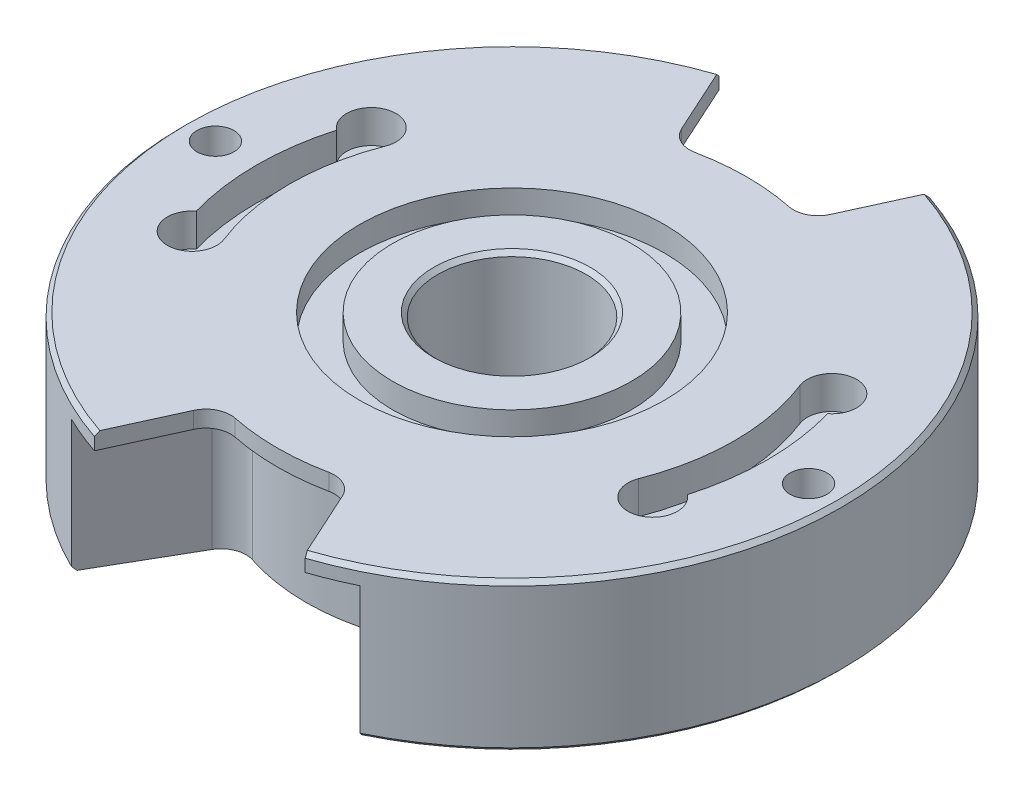
SolidWorks part; units mm, degrees
ref_plane "Front Plane" through (0, 0, 0) normal (0, 0, 1) x (1, 0, 0)
ref_plane "Top Plane" through (0, 0, 0) normal (0, 1, 0) x (1, 0, 0)
ref_plane "Right Plane" through (0, 0, 0) normal (1, 0, 0) x (0, 0, -1)
other "Configuration Table"
sketch "Sketch1" plane through (0, 0, 0) normal (0, 1, 0) x (1, 0, 0)
  circle A0 centre (0, 0) radius 40
  dimension "D1" = 80
extrude "Boss-Extrude1" add sketch "Sketch1" along normal blind 18
chamfer "Chamfer2" distance 0.5 angle 45 2 edges at (0, 0, 40) (0, 18, 40)
sketch "Sketch2" plane through (0, 18, 0) normal (0, 1, 0) x (1, 0, 0)
  line L0 (-36, 0) -> (36, 0) construction
  line L1 (0, 0) -> (0, -31.9265) construction
  circle A0 centre (36, 0) radius 2.25
  circle A1 centre (-36, 0) radius 2.25
  dimension "D1" = 4.5
  dimension "D2" = 36
extrude "Cut-Extrude1" cut sketch "Sketch2" against normal through all and the other way through all
sketch "Sketch3" plane through (0, 18, 0) normal (0, 1, 0) x (1, 0, 0)
  line L0 (-54.6069, 0) -> (54.6069, 0) construction
  line L1 (0, 0) -> (-45.6722, 23.2711) construction
  line L2 (0, 0) -> (-45.6722, -23.2711) construction
  line L3 (0, 0) -> (0, 53.5192) construction
  line L4 (0, 0) -> (45.6722, -23.2711) construction
  line L5 (0, 0) -> (45.6722, 23.2711) construction
  arc A0 (-25.1624, 9.7906) -> (-25.1624, -9.7906) centre (0, 0) ccw
  arc A2 (-25.1624, 9.7906) -> (-29.8073, 8.5161) centre (-27.9582, 10.8784) ccw
  arc A3 (-29.8073, 8.5161) -> (-29.8073, -8.5161) centre (0, 0) ccw
  arc A4 (-25.1624, -9.7906) -> (-29.8073, -8.5161) centre (-27.9582, -10.8784) cw
  arc A5 (25.1624, -9.7906) -> (29.8073, -8.5161) centre (27.9582, -10.8784) ccw
  arc A6 (29.8073, 8.5161) -> (29.8073, -8.5161) centre (0, 0) cw
  arc A7 (25.1624, 9.7906) -> (29.8073, 8.5161) centre (27.9582, 10.8784) cw
  arc A8 (25.1624, 9.7906) -> (25.1624, -9.7906) centre (0, 0) cw
  dimension "D1" = 54
  dimension "D2" = 31
  dimension "D4" = 6
  dimension "D3" = 27
extrude "Cut-Extrude2" cut sketch "Sketch3" against normal blind 4
sketch "Sketch4" plane through (0, 18, 0) normal (0, 1, 0) x (1, 0, 0)
  line L0 (0, 64.1872) -> (0, 0) construction
  line L1 (-12.7978, 37.8975) -> (-9.0257, 29.6204)
  line L2 (0, 0) -> (-60.0977, 0) construction
  line L3 (12.7978, 37.8975) -> (9.0257, 29.6204)
  line L4 (12.7978, -37.8975) -> (9.0257, -29.6204)
  line L5 (-12.7978, -37.8975) -> (-9.0257, -29.6204)
  arc A0 (5.6962, 27.925) -> (-5.6962, 27.925) centre (0, 0) ccw
  circle A1 centre (0, 0) radius 40 construction
  arc A3 (-25.1624, 9.7906) -> (-29.8073, 8.5161) centre (-27.9582, 10.8784) ccw construction
  arc A4 (12.7978, 37.8975) -> (-12.7978, 37.8975) centre (0, 0) ccw
  arc A5 (9.0257, 29.6204) -> (5.6962, 27.925) centre (6.2958, 30.8644) cw
  arc A6 (-9.0257, 29.6204) -> (-5.6962, 27.925) centre (-6.2958, 30.8644) ccw
  arc A7 (-9.0257, -29.6204) -> (-5.6962, -27.925) centre (-6.2958, -30.8644) cw
  arc A8 (9.0257, -29.6204) -> (5.6962, -27.925) centre (6.2958, -30.8644) ccw
  arc A9 (12.7978, -37.8975) -> (-12.7978, -37.8975) centre (0, 0) cw
  arc A10 (5.6962, -27.925) -> (-5.6962, -27.925) centre (0, 0) cw
  point P14 (7.9937, 27.356)
  point P17 (-7.9937, 27.356)
  point P26 (-7.9937, -27.356)
  point P27 (7.9937, -27.356)
  dimension "D1" = 57
  dimension "D3" = 25
  dimension "D4" = 3
  dimension "D2" = 24.5
extrude "Cut-Extrude3" cut sketch "Sketch4" against normal through all
sketch "Sketch5" plane through (0, 0, 0) normal (0, -1, 0) x (-1, 0, 0)
  circle A0 centre (0, 0) radius 9
  dimension "D1" = 18
extrude "Cut-Extrude4" cut sketch "Sketch5" against normal through all
sketch "Sketch6" plane through (0, 0, 0) normal (0, -1, 0) x (-1, 0, 0)
  line L0 (57.0258, 0) -> (0, 0) construction
  line L1 (0, 60.3123) -> (0, -60.3123) construction
  line L2 (17.5295, -35.9544) -> (11.2752, -25.1216)
  line L5 (-17.5295, -35.9544) -> (-11.2752, -25.1216)
  line L6 (-17.5295, 35.9544) -> (-11.2752, 25.1216)
  line L7 (17.5295, 35.9544) -> (11.2752, 25.1216)
  arc A0 (-7.7474, -23.7693) -> (7.7474, -23.7693) centre (0, 0) ccw
  arc A2 (-20.2055, 34.5216) -> (-20.2055, -34.5216) centre (0, 0) ccw construction
  arc A3 (-17.5295, -35.9544) -> (17.5295, -35.9544) centre (0, 0) ccw
  arc A4 (-17.5295, 35.9544) -> (17.5295, 35.9544) centre (0, 0) cw
  arc A5 (-7.7474, 23.7693) -> (7.7474, 23.7693) centre (0, 0) cw
  arc A6 (-11.2752, -25.1216) -> (-7.7474, -23.7693) centre (-8.6771, -26.6216) cw
  arc A7 (11.2752, -25.1216) -> (7.7474, -23.7693) centre (8.6771, -26.6216) ccw
  arc A8 (7.7474, 23.7693) -> (11.2752, 25.1216) centre (8.6771, 26.6216) ccw
  arc A9 (-7.7474, 23.7693) -> (-11.2752, 25.1216) centre (-8.6771, 26.6216) cw
  point P18 (-10, -22.9129)
  point P21 (10, -22.9129)
  point P24 (10, 22.9129)
  point P27 (-10, 22.9129)
  dimension "D1" = 50
  dimension "D3" = 3
  dimension "D2" = 30
  dimension "D4" = 10
extrude "Cut-Extrude5" cut sketch "Sketch6" against normal blind 16
sketch "Sketch7" plane through (0, 18, 0) normal (0, 1, 0) x (1, 0, 0)
  circle A0 centre (0, 0) radius 14.5
  circle A1 centre (0, 0) radius 18.5
  dimension "D1" = 29
  dimension "D2" = 37
extrude "Cut-Extrude6" cut sketch "Sketch7" against normal blind 3
chamfer "Chamfer1" distance 0.5 angle 45 2 edges at (0, 0, -9) (0, 18, -9)
